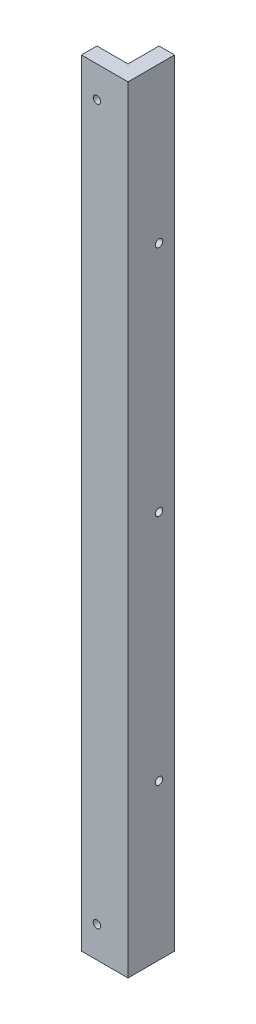
from build123d import *

# Parameters (mm, degrees)
BOSS_EXTRUDE1_DEPTH = 250
SKETCH3_R           = 1.2
CUT_EXTRUDE1_DEPTH  = 10
SKETCH4_R           = 1.2
CUT_EXTRUDE2_DEPTH  = 5


with BuildPart() as part:
    # Sketch1 → Boss-Extrude1 (new body)
    with BuildSketch(Plane(origin=(0, 0, 0), x_dir=(1, 0, 0), z_dir=(0, 1, 0))):
        Polygon((0, 0), (15, 0), (15, 15), (10, 15), (10, 5), (0, 5), align=None)
    extrude(amount=BOSS_EXTRUDE1_DEPTH)

    # Sketch3 → Cut-Extrude1 (cut)
    with BuildSketch(Plane.ZY.offset(-10)):
        with Locations((-10, 50)):
            Circle(SKETCH3_R)
        with Locations((-10, 125)):
            Circle(SKETCH3_R)
        with Locations((-10, 200)):
            Circle(SKETCH3_R)
    extrude(amount=-CUT_EXTRUDE1_DEPTH, mode=Mode.SUBTRACT)

    # Sketch4 → Cut-Extrude2 (cut)
    with BuildSketch(Plane.XY):
        with Locations((5, 10)):
            Circle(SKETCH4_R)
        with Locations((5, 240)):
            Circle(SKETCH4_R)
    extrude(amount=-CUT_EXTRUDE2_DEPTH, mode=Mode.SUBTRACT)


solid = part.part
